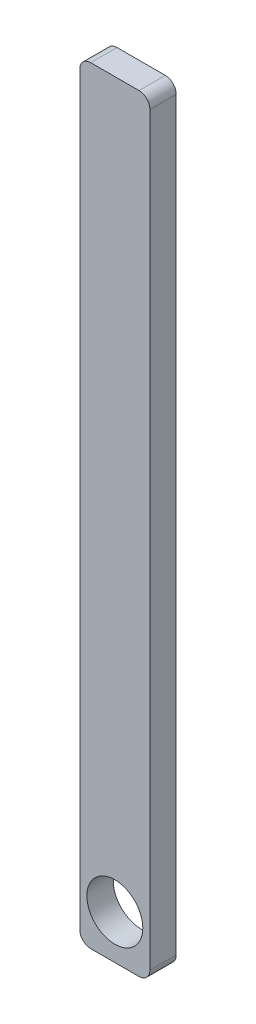
SolidWorks part; units mm, degrees
material "AISI 1045 钢，冷拔"
ref_plane "Front Plane" through (0, 0, 0) normal (0, 0, 1) x (1, 0, 0)
ref_plane "Top Plane" through (0, 0, 0) normal (0, 1, 0) x (1, 0, 0)
ref_plane "Right Plane" through (0, 0, 0) normal (1, 0, 0) x (0, 0, -1)
sketch "Sketch1" plane through (0, 0, 0) normal (0, 0, 1) x (1, 0, 0)
  line L1 (5, 0) -> (27, 0)
  line L2 (0, 5) -> (0, 345)
  line L3 (5, 350) -> (27, 350)
  line L4 (32, 5) -> (32, 345)
  arc A0 (27, 0) -> (32, 5) centre (27, 5) ccw
  arc A1 (0, 345) -> (5, 350) centre (5, 345) cw
  arc A2 (27, 350) -> (32, 345) centre (27, 345) cw
  arc A3 (5, 0) -> (0, 5) centre (5, 5) cw
  circle A4 centre (16, 20) radius 12.75
  point P7 (32, 0)
  point P10 (0, 350)
  point P15 (0, 0)
  dimension "D3" = 5
  dimension "D4" = 25.5
  dimension "D6" = 16
  dimension "D1" = 350
  dimension "D2" = 32
  dimension "D5" = 20
extrude "Boss-Extrude1" add sketch "Sketch1" along normal blind 12
